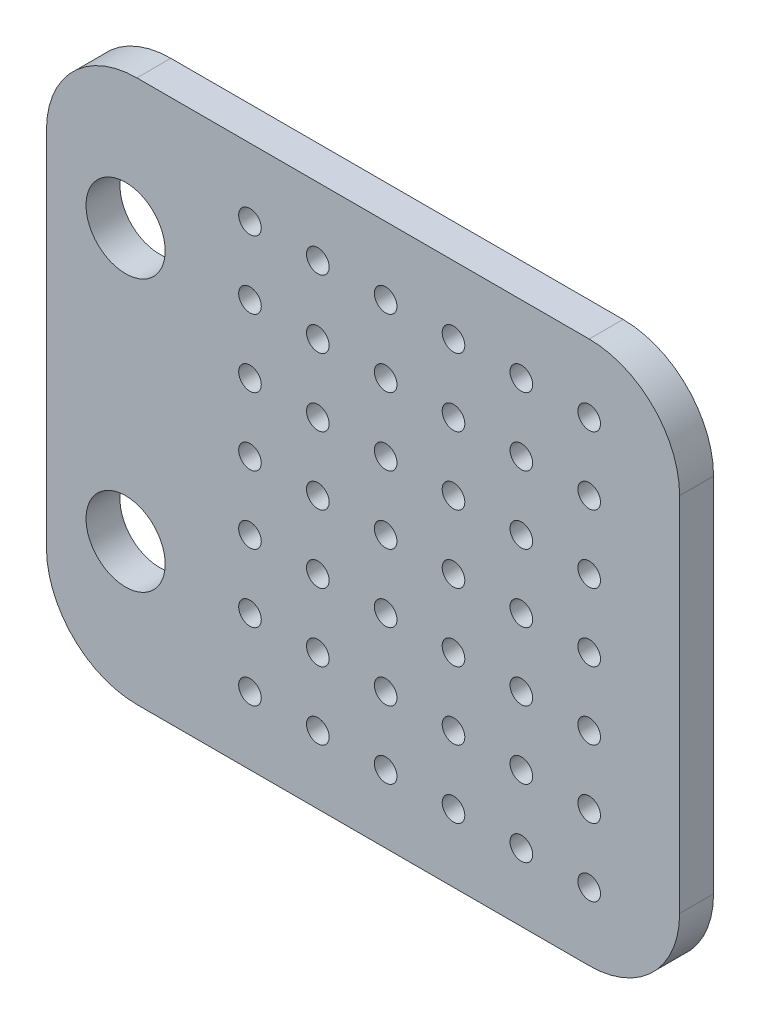
SolidWorks part; units mm, degrees
ref_plane "Front Plane" through (0, 0, 0) normal (0, 0, 1) x (1, 0, 0)
ref_plane "Top Plane" through (0, 0, 0) normal (0, 1, 0) x (1, 0, 0)
ref_plane "Right Plane" through (0, 0, 0) normal (1, 0, 0) x (0, 0, -1)
sketch "Sketch1" plane through (0, 0, 0) normal (0, 0, 1) x (1, 0, 0)
  line L1 (-14, 12) -> (14, 12)
  line L2 (-14, 12) -> (-14, -12)
  line L3 (-14, -12) -> (14, -12)
  line L4 (14, 12) -> (14, -12)
  line L5 (-14, 12) -> (14, -12) construction
  line L6 (-14, -12) -> (14, 12) construction
  point P0 (0, 0)
  dimension "D1" = 28
  dimension "D2" = 24
extrude "Boss-Extrude1" add sketch "Sketch1" along normal mid plane 1.5
fillet "Fillet1" radius 4 4 edges at (-14, -12, 0) (14, -12, 0) (-14, 12, 0) (14, 12, 0)
hole_wizard "Ø3.5 (3.5) Diameter Hole1" positions "Sketch3" profile "Sketch2" hole size "Ø3.5" standard "Gb" end condition through all
sketch "Sketch3" plane through (0, 0, 0.75) normal (0, 0, 1) x (1, 0, 0)
  line L0 (0, 0) -> (17.7701, 0) construction
  line L3 (-14, 8) -> (-14, -8) construction
  point P0 (-10.5, 6)
  point P2 (-10.5, -6)
  dimension "D1" = 12
  dimension "D2" = 3.5
sketch "Sketch2" plane through (-10.5, 6, 0.75) normal (1, 0, 0) x (0, -1, 0)
  line L0 (0, 0) -> (0, 1.5)
  line L1 (0, 1.5) -> (1.75, 1.5)
  line L2 (1.75, 1.5) -> (1.75, 0)
  line L5 (1.75, 0) -> (0, 0)
  line L11 (0, -6.35) -> (0, 107.95) construction
  dimension "通孔孔直径" = 3.5
  dimension "通孔孔深度" = 1.5
hole_wizard "Ø1.0 (1) Diameter Hole1" positions "Sketch6" profile "Sketch5" hole size "Ø1.0" standard "Gb" end condition through all
sketch "Sketch6" plane through (0, 0, 0.75) normal (0, 0, 1) x (1, 0, 0)
  line L0 (14, -8) -> (14, 8) construction
  line L1 (-10, -12) -> (10, -12) construction
  point P0 (10, -9)
  dimension "D1" = 4
  dimension "D2" = 3
sketch "Sketch5" plane through (10, -9, 0.75) normal (1, 0, 0) x (0, -1, 0)
  line L0 (0, 0) -> (0, 1.5)
  line L1 (0, 1.5) -> (0.5, 1.5)
  line L2 (0.5, 1.5) -> (0.5, 0)
  line L5 (0.5, 0) -> (0, 0)
  line L11 (0, -6.35) -> (0, 107.95) construction
  dimension "通孔孔直径" = 1
  dimension "通孔孔深度" = 1.5
pattern_linear "LPattern1" count 6 spacing 3 along (-1, 0, 0) count 7 spacing 3 along (0, 1, 0) of "Ø1.0 (1) Diameter Hole1"
